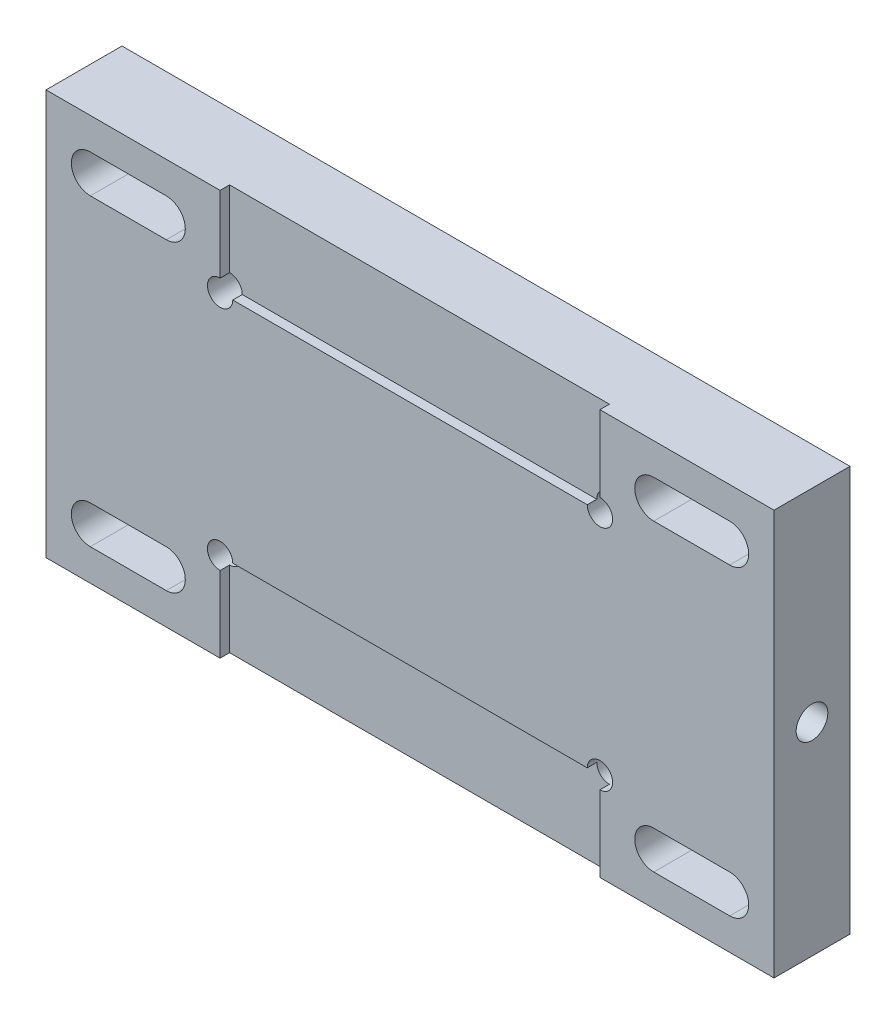
from build123d import *

# Parameters (mm, degrees)
SKETCH_1_W             = 115
SKETCH_1_H             = 64
EXTRUDE_1_DEPTH        = 6
SKETCH_2_W             = 60
SKETCH_2_H             = 14
CUT_EXTRUDE_1_DEPTH    = 1.5
SKETCH_3_R             = 2
CUT_EXTRUDE_2_DEPTH    = 67.889834803
CUT_EXTRUDE_3_REACH    = 68.89
HOLE_WIZARD_M6_1_D     = 5
HOLE_WIZARD_M6_1_DEPTH = 18
HOLE_WIZARD_M6_1_TIP   = 1.502151548


with BuildPart() as part:
    # 草图1 → 凸台-拉伸1 (new, symmetric)
    with BuildSketch(Plane.XY):
        Rectangle(SKETCH_1_W, SKETCH_1_H)
    extrude(amount=EXTRUDE_1_DEPTH, both=True)

    # 草图2 → 切除-拉伸1 (cut)
    with BuildSketch(Plane.XY.offset(6)):
        with Locations((0, 25)):
            Rectangle(SKETCH_2_W, SKETCH_2_H)
    cut_extrude_1 = extrude(amount=-CUT_EXTRUDE_1_DEPTH, mode=Mode.SUBTRACT)

    # 草图3 → 切除-拉伸2 (cut, symmetric)
    with BuildSketch(Plane.XY.offset(6)):
        with Locations((-30, 18)):
            Circle(SKETCH_3_R)
        with Locations((30, 18)):
            Circle(SKETCH_3_R)
    cut_extrude_2 = extrude(amount=CUT_EXTRUDE_2_DEPTH, both=True, mode=Mode.SUBTRACT)

    # 镜向1: 切除-拉伸1, 切除-拉伸2 across plane
    add(cut_extrude_1.mirror(Plane.ZX), mode=Mode.SUBTRACT)
    add(cut_extrude_2.mirror(Plane.ZX), mode=Mode.SUBTRACT)

    # 草图4 → 切除-拉伸3 (cut, up to next)
    with BuildSketch(Plane.XY.offset(6), mode=Mode.PRIVATE) as cut_extrude_3_sk1:
        with BuildLine():
            Line((-50.5, 27), (-38.5, 27))
            ThreePointArc((-38.5, 27), (-35.5, 24), (-38.5, 21))
            Line((-38.5, 21), (-50.5, 21))
            ThreePointArc((-50.5, 21), (-53.5, 24), (-50.5, 27))
        make_face()
    cut_extrude_3_tool1 = extrude(cut_extrude_3_sk1.sketch, amount=-CUT_EXTRUDE_3_REACH, mode=Mode.PRIVATE) & part.part
    # 草图4 → 切除-拉伸3 (cut, up to next)
    with BuildSketch(Plane.XY.offset(6), mode=Mode.PRIVATE) as cut_extrude_3_sk2:
        with BuildLine():
            Line((50.5, 27), (38.5, 27))
            ThreePointArc((38.5, 27), (35.5, 24), (38.5, 21))
            Line((38.5, 21), (50.5, 21))
            ThreePointArc((50.5, 21), (53.5, 24), (50.5, 27))
        make_face()
    cut_extrude_3_tool2 = extrude(cut_extrude_3_sk2.sketch, amount=-CUT_EXTRUDE_3_REACH, mode=Mode.PRIVATE) & part.part
    # 草图4 → 切除-拉伸3 (cut, up to next)
    with BuildSketch(Plane.XY.offset(6), mode=Mode.PRIVATE) as cut_extrude_3_sk3:
        with BuildLine():
            Line((-50.5, -27), (-38.5, -27))
            ThreePointArc((-38.5, -27), (-35.5, -24), (-38.5, -21))
            Line((-38.5, -21), (-50.5, -21))
            ThreePointArc((-50.5, -21), (-53.5, -24), (-50.5, -27))
        make_face()
    cut_extrude_3_tool3 = extrude(cut_extrude_3_sk3.sketch, amount=-CUT_EXTRUDE_3_REACH, mode=Mode.PRIVATE) & part.part
    # 草图4 → 切除-拉伸3 (cut, up to next)
    with BuildSketch(Plane.XY.offset(6), mode=Mode.PRIVATE) as cut_extrude_3_sk4:
        with BuildLine():
            Line((50.5, -27), (38.5, -27))
            ThreePointArc((38.5, -27), (35.5, -24), (38.5, -21))
            Line((38.5, -21), (50.5, -21))
            ThreePointArc((50.5, -21), (53.5, -24), (50.5, -27))
        make_face()
    cut_extrude_3_tool4 = extrude(cut_extrude_3_sk4.sketch, amount=-CUT_EXTRUDE_3_REACH, mode=Mode.PRIVATE) & part.part
    add(cut_extrude_3_tool1.solids().sort_by_distance((-44.5, 24, 6))[0], mode=Mode.SUBTRACT)
    add(cut_extrude_3_tool2.solids().sort_by_distance((44.5, 24, 6))[0], mode=Mode.SUBTRACT)
    add(cut_extrude_3_tool3.solids().sort_by_distance((-44.5, -24, 6))[0], mode=Mode.SUBTRACT)
    add(cut_extrude_3_tool4.solids().sort_by_distance((44.5, -24, 6))[0], mode=Mode.SUBTRACT)

    # M6 螺纹孔1
    with Locations(Plane(origin=(57.5, 0, 0), x_dir=(0, 0, 1), z_dir=(1, 0, 0))):
        with Locations((0, 0)):
            Hole(HOLE_WIZARD_M6_1_D / 2, depth=HOLE_WIZARD_M6_1_DEPTH)
            with Locations((0, 0, -(HOLE_WIZARD_M6_1_DEPTH + HOLE_WIZARD_M6_1_TIP / 2))):  # 118° drill point
                Cone(0, HOLE_WIZARD_M6_1_D / 2, HOLE_WIZARD_M6_1_TIP, mode=Mode.SUBTRACT)


solid = part.part
